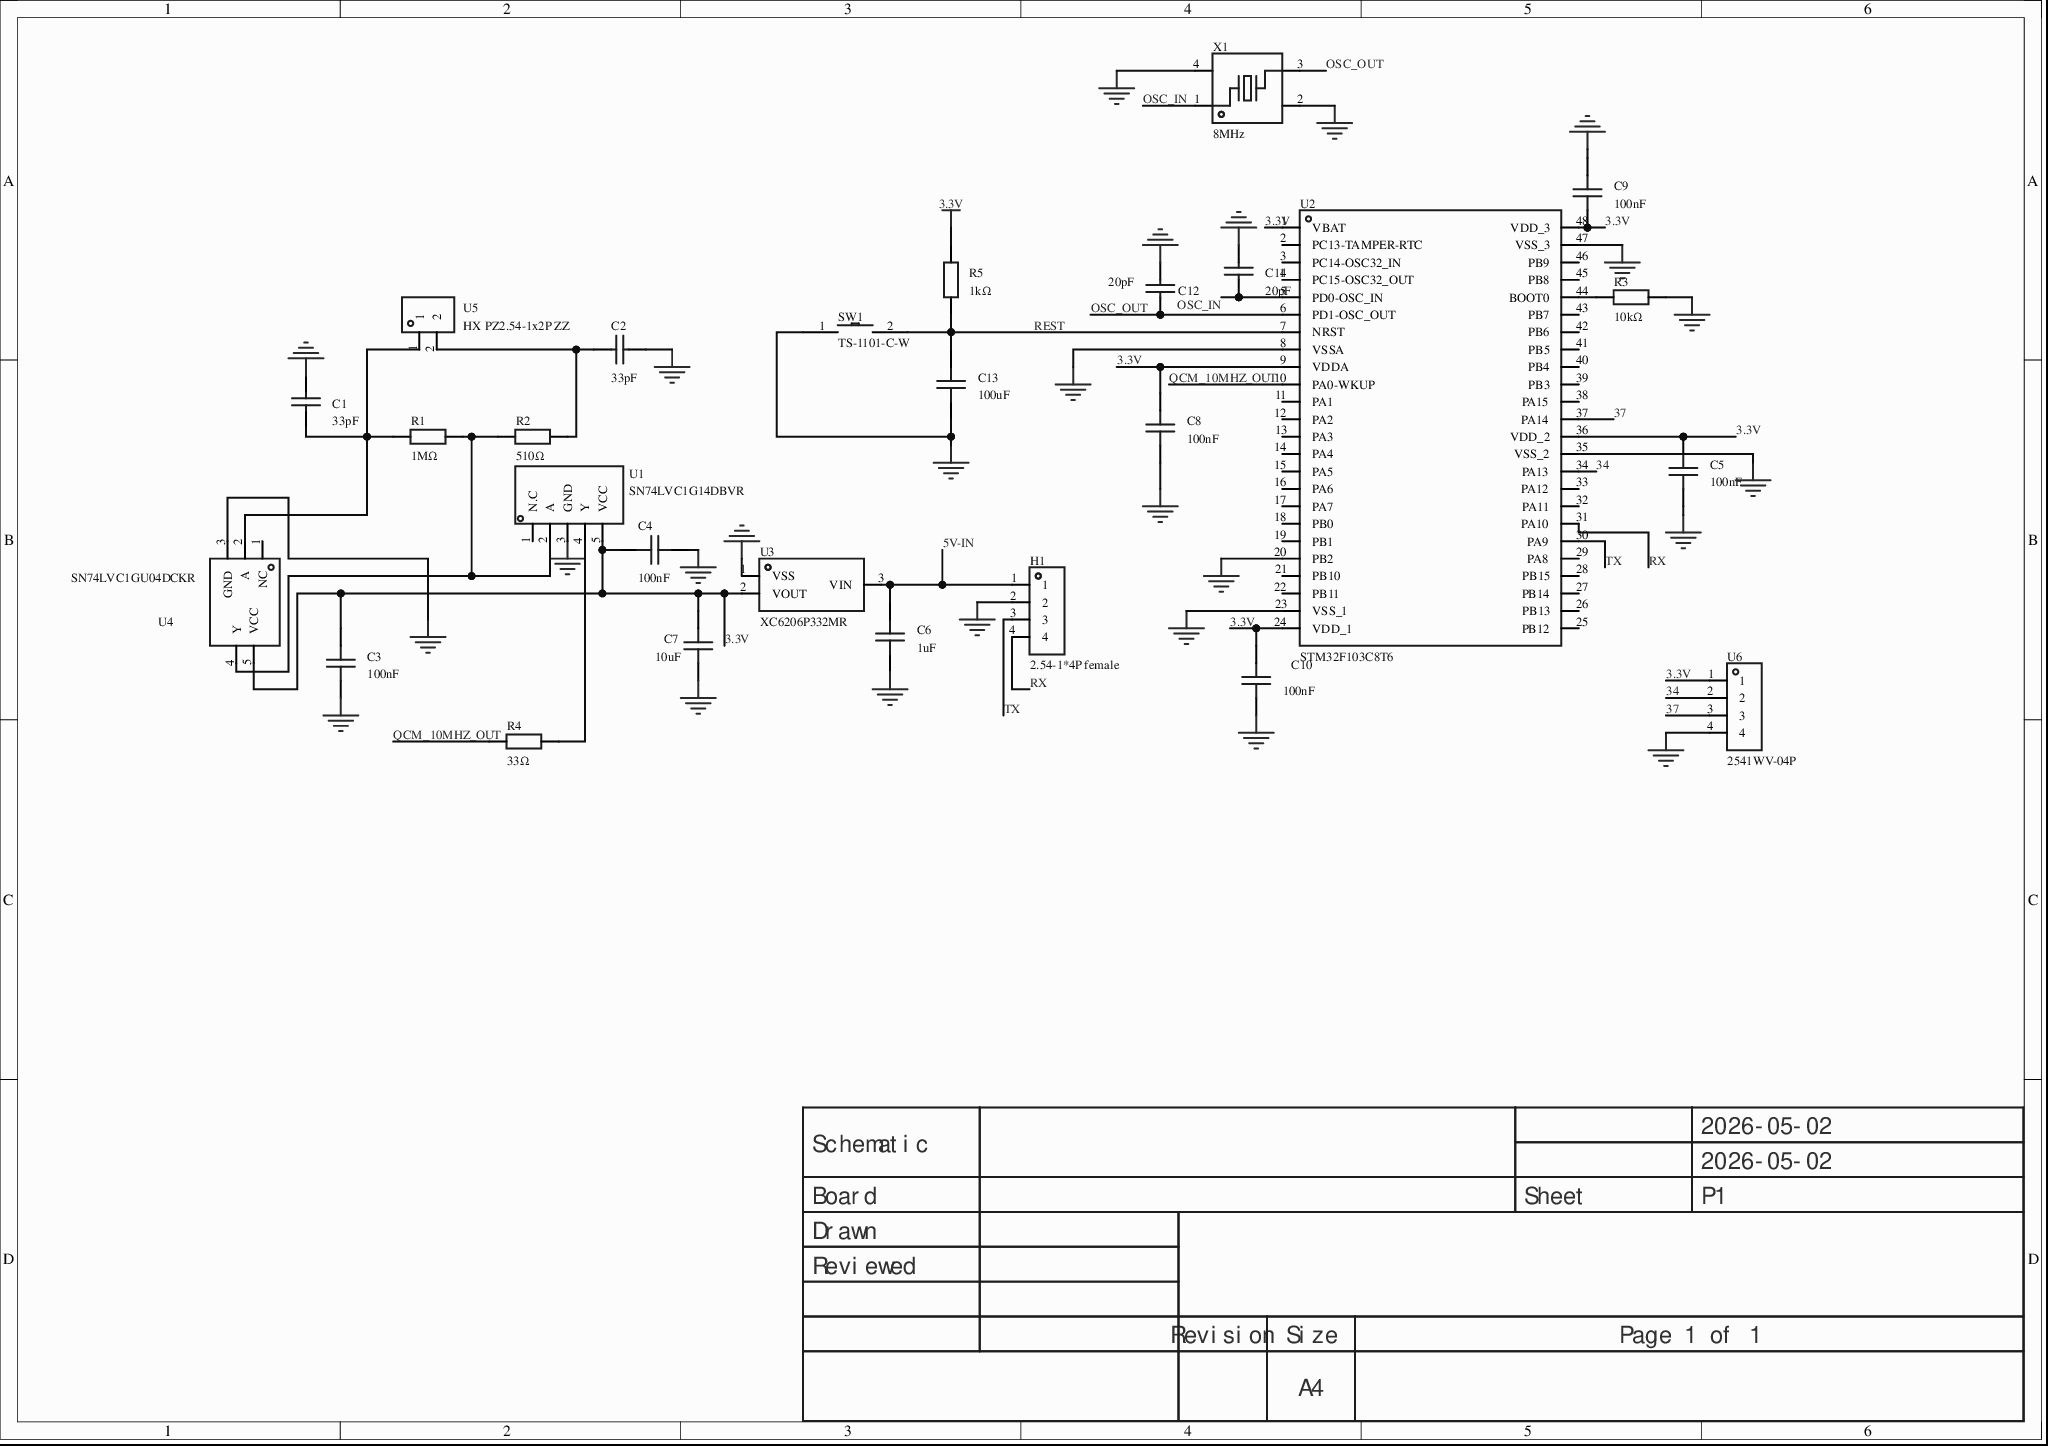
[diagram p0: MISC51896-3.schdoc]
# Altium project MISC51896-2.PrjPcb
1 sheet, 27 parts. Net scope: global (net labels, ports and power ports of the same name join across sheets).
Board file: MISC51896.pcbdoc

## Sheet MISC51896-3.schdoc
size 297 x 209 mm; Version: V1.0; @Project Name: MISC51896; @Update Date: 2026-05-02; @Create Date: 2026-05-02; @Board Name: MISC51896; @Create Time: 19:24:28; @Page Count: 1; @Page No: 1; @Schematic Name: MISC51896; @Update Time: 19:24:28; Size: A4

### Parts
C1  33pF  [C0603]
C2  33pF  [C0603]
C3  100nF  [C0603]
C4  100nF  [C0603]
C5  100nF  [C0603]
C6  1uF  [C0603]
C7  10uF  [C0603]
C8  100nF  [C0603]
C9  100nF  [C0603]
C10  100nF  [C0603]
C11  20pF  [C0603]
C12  20pF  [C0603]
C13  100uF  [C1206]
H1  2.54-1*4P female  [HDR-TH_4P-P2.54-V-F]
R1  1MΩ  [R0603]
R2  510Ω  [R0603]
R3  10kΩ  [R0603]
R4  33Ω  [R0603]
R5  1kΩ  [R0603]
SW1  TS-1101-C-W  [SW-SMD_L6.0-W3.3-LS8.0]
U1  SN74LVC1G14DBVR  [SOT-23-5_L3.0-W1.7-P0.95-LS2.8-BR]
U2  STM32F103C8T6  [LQFP-48_L7.0-W7.0-P0.50-LS9.0-BL]
U3  XC6206P332MR  [SOT-23-3_L3.0-W1.7-P0.95-LS2.9-BR]
U4  SN74LVC1GU04DCKR  [SC-70-5_L2.1-W1.3-P0.65-LS2.1-BL]
U5  HX PZ2.54-1x2P ZZ  [HDR-TH_2P-P2.54-V-M-3]
U6  2541WV-04P  [HDR-TH_4P-P2.54-V-M-1]
X1  8MHz  [CRYSTAL-SMD_4P-L3.2-W2.5-BL]

### Nets
3.3V: C3.2 C4.1 C5.2 C7.2 C8.2 C9.1 C10.2 R5.2 U1.5(VCC) U2.1(VBAT) U2.9(VDDA) U2.24(VDD_1) U2.36(VDD_2) U2.48(VDD_3) U3.2(VOUT) U4.5(VCC) U6.1
GND: C1.2 C2.2 C3.1 C4.2 C5.1 C6.1 C7.1 C8.1 C9.2 C10.1 C11.2 C12.2 C13.1 H1.2 R3.2 SW1.1 U1.3(GND) U2.8(VSSA) U2.20(PB2) U2.23(VSS_1) U2.35(VSS_2) U2.47(VSS_3) U3.1(VSS) U4.3(GND) U6.4 X1.2(GND) X1.4(GND)
5V-IN: C6.2 H1.1 U3.3(VIN)
34: U2.34(PA13) U6.2
37: U2.37(PA14) U6.3
OSC_IN: C11.1 U2.5(PD0-OSC_IN) X1.1
OSC_OUT: C12.1 U2.6(PD1-OSC_OUT) X1.3
QCM_10MHZ_OUT: R4.1 U2.10(PA0-WKUP)
REST: C13.2 R5.1 SW1.2 U2.7(NRST)
RX: H1.4 U2.31(PA10)
TX: H1.3 U2.30(PA9)
NetC1_1: C1.1 R1.1 U4.2(A) U5.1
NetC2_1: C2.1 R2.2 U5.2
NetR1_2: R1.2 R2.1 U1.2(A) U4.4(Y)
NetR3_1: R3.1 U2.44(BOOT0)
NetR4_2: R4.2 U1.4(Y)

Not connected (* = marked no-connect by the designer): U1 1(N.C); U2 2(PC13-TAMPER-RTC) 3(PC14-OSC32_IN) 4(PC15-OSC32_OUT) 11(PA1) 12(PA2) 13(PA3) 14(PA4) 15(PA5) 16(PA6) 17(PA7) 18(PB0) 19(PB1) 21(PB10) 22(PB11) 25(PB12) 26(PB13) 27(PB14) 28(PB15) 29(PA8) 32(PA11) 33(PA12) 38(PA15) 39(PB3) 40(PB4) 41(PB5) 42(PB6) 43(PB7) 45(PB8) 46(PB9); U4 1(NC)

### Notes on the sheet
- 2026-05-02
- Schematic
- Board
- Sheet
- P1
- Drawn
- Reviewed
- Revision
- Size
- A4
- Page 1 of 1

### Library data of the parts
C1 C2 = CL10C330JB8NNNC: Capacitance:33pF;Tolerance:±5%;Rated voltage:50V;Temperature coefficient:C0G;; Manufacturer: SAMSUNG(三星); AddInBom: yes; ModelId: ac125912035d415993ca9572d50418b10819f05c4eef4c71ace90d822a990e87; ModelName: C0603_L1.6-W0.8-H0.8; ModelTransform: 62.992,31.496,0,0,0,0,0,0,0; Tolerance: ±5%; Voltage Rating: 50V; Temperature Coefficient: C0G; Symbol: CL10C330JB8NNNC; Device: CL10C330JB8NNNC; LCSC Part Name: 33pF ±5% 50V; SupplierPart: C1663; ManufacturerPart: CL10C330JB8NNNC; Supplier Footprint: 0603; JLCPCB Part Class: Basic Part; Datasheet: https://item.szlcsc.com/datasheet/CL10C330JB8NNNC/2015.html; Supplier: LCSC; ConvertToPcb: yes; FootprintName: C0603; Value: 33pF
C3 C4 = CGA0603X7R104K500JT: Capacitance:100nF;Tolerance:±10%;Rated voltage:50V;Temperature coefficient:X7R;; Manufacturer: HRE(芯声); AddInBom: yes; ModelId: ac125912035d415993ca9572d50418b10819f05c4eef4c71ace90d822a990e87; ModelName: C0603_L1.6-W0.8-H0.8; ModelTransform: 62.992,31.496,0,0,0,0,0,0,0; Tolerance: ±10%; Voltage Rating: 50V; Temperature Coefficient: X7R; Symbol: CGA0603X7R104K500JT; Device: CGA0603X7R104K500JT; LCSC Part Name: 100nF ±10% 50V; SupplierPart: C6119867; ManufacturerPart: CGA0603X7R104K500JT; Supplier Footprint: 0603; JLCPCB Part Class: Extended Part; Datasheet: https://item.szlcsc.com/datasheet/CGA0603X7R104K500JT/7062573.html; Supplier: LCSC; ConvertToPcb: yes; FootprintName: C0603; Value: 100nF
C5 C8-C10 = CGA0603X7R104K500JT: Capacitance:100nF;Tolerance:±10%;Rated voltage:50V;Temperature coefficient:X7R;; Manufacturer: HRE(芯声); Add into BOM: yes; 3D Model: ac125912035d415993ca9572d50418b1; 3D Model Transform: 62.992,31.496,0,0,0,0,0,0,0; Tolerance: ±10%; Voltage Rating: 50V; Temperature Coefficient: X7R; ModelName: C0603_L1.6-W0.8-H0.8; Symbol: CGA0603X7R104K500JT; Device: CGA0603X7R104K500JT; Convert to PCB: yes; LCSC Part Name: 100nF ±10% 50V; Supplier Part: C6119867; Manufacturer Part: CGA0603X7R104K500JT; Supplier Footprint: 0603; JLCPCB Part Class: Extended Part; Datasheet: https://item.szlcsc.com/datasheet/CGA0603X7R104K500JT/7062573.html; Supplier: LCSC; Value: 100nF; FootprintName: C0603
C6 C7 = CGA0603X5R105K500JT: Capacitance:1uF;Tolerance:±10%;Rated voltage:50V;Temperature coefficient:X5R;; Manufacturer: HRE(芯声); AddInBom: yes; ModelId: ac125912035d415993ca9572d50418b10819f05c4eef4c71ace90d822a990e87; ModelName: C0603_L1.6-W0.8-H0.8; ModelTransform: 62.992,31.496,0,0,0,0,0,0,0; Tolerance: ±10%; Voltage Rating: 50V; Temperature Coefficient: X5R; Symbol: CGA0603X5R105K500JT; Device: CGA0603X5R105K500JT; LCSC Part Name: 1uF ±10% 50V; ManufacturerPart: CGA0603X5R105K500JT; Supplier Footprint: 0603; JLCPCB Part Class: Extended Part; Datasheet: https://item.szlcsc.com/datasheet/CGA0603X5R105K500JT/7062558.html; Supplier: LCSC; ConvertToPcb: yes; FootprintName: C0603
  C6: SupplierPart: C6119852; Value: 1uF
  C7: Value: 10uF
C11 C12 = CL10C200JB8NNNC: Capacitance:20pF;Tolerance:±5%;Rated voltage:50V;Temperature coefficient:C0G;; Manufacturer: SAMSUNG(三星); Add into BOM: yes; 3D Model: ac125912035d415993ca9572d50418b1; 3D Model Transform: 62.992,31.496,0,0,0,0,0,0,0; Tolerance: ±5%; Voltage Rating: 50V; Temperature Coefficient: C0G; ModelName: C0603_L1.6-W0.8-H0.8; Symbol: CL10C200JB8NNNC; Device: CL10C200JB8NNNC; Convert to PCB: yes; Supplier Footprint: 0603; Value: 20pF; LCSC Part Name: 20pF ±5% 50V; Supplier Part: C1648; Manufacturer Part: CL10C200JB8NNNC; JLCPCB Part Class: Basic Part; Datasheet: https://item.szlcsc.com/datasheet/CL10C200JB8NNNC/2000.html; Supplier: LCSC; FootprintName: C0603
C13 = HGC1206R5107M100NSPJ: Capacitance:100uF;Tolerance:±20%;Rated voltage:10V;Dielectric (temperature coefficient):X5R;; Manufacturer: Chinocera(华瓷); 3D Model: e4be705b945545a48e666415e3682bd8; 3D Model Transform: 125.984,62.992,0,0,0,0,0,0,0; Tolerance: ±20%; Voltage Rated: 10V; Temperature Coefficient: X5R; AddInBom: yes; ModelName: C1206_L3.2-W1.6-H1.3; Symbol: HGC1206R5107M100NSPJ; Device: HGC1206R5107M100NSPJ; LCSC Part Name: 100uF ±20% 10V; Supplier Part: C7432784; Manufacturer Part: HGC1206R5107M100NSPJ; Supplier Footprint: 1206; JLCPCB Part Class: Extended library; Datasheet: https://atta.szlcsc.com/upload/public/pdf/source/20240320/FAC3FEC40A78BC5CCCE96C232A94D860.pdf; Supplier: LCSC; Value: 100uF; ConvertToPcb: yes; FootprintName: C1206
H1 = 2.54-1*4P母: Socket structure:1x4P;Pitch:2.54mm;Row spacing:-;Round/square hole:square hole;Mounting:through-hole;Rows:single row;Total holes:4P;Rated current:3A;Rated voltage:-;Socket direction:top;Plastic height:-;Contact material:Bronze;Contact plating:-;Operating temperature:-40℃~+105℃;; Manufacturer: BOOMELE(博穆精密); AddInBom: yes; ModelId: d187812051054f85879fcaa51a310d8e0819f05c4eef4c71ace90d822a990e87; ModelTransform: 419.6842,98.464,0,0,0,0,0,0,-118.11; Holes Structure: 1x4P; Pitch: 2.54mm; Number of Positions: 4P; Current Rating: 3A; Holes Direction: Top; Symbol: 2.54-1*4P female; Device: 2.54-1*4P female; LCSC Part Name: 间距:2.54mm 1x4P 直插; SupplierPart: C2718488; ManufacturerPart: 2.54-1*4P母; Supplier Footprint: 插件,P=2.54mm; JLCPCB Part Class: Extended Part; Datasheet: https://item.szlcsc.com/datasheet/2.54-1*4P%25E6%25AF%258D/2834502.html; Supplier: LCSC; ConvertToPcb: yes; FootprintName: HDR-TH_4P-P2.54-V-F; ModelName: HDR-TH_4P-P2.54-V-F; Row Spacing: -; Circular Hole / Square Hole: Square hole; Mounting Type: Through-hole; Number of Rows: Single row; Voltage Rating (Max): -; Insulation Height: -; Contact Material: Bronze; Contact Plating: -; Operating Temperature: -40℃~+105℃
R1 = 0603WAF1004T5E: Resistor type:thick film;Resistance:1MΩ;Tolerance:±1%;Power:100mW;Max working voltage:75V;Temperature coefficient:±100ppm/℃;; Manufacturer: UNI-ROYAL(厚声); AddInBom: yes; ModelId: fc143cca1e79419f9cd78b61e9279f080819f05c4eef4c71ace90d822a990e87; ModelTransform: 31.8897,63.7794,0,90,0,0,0,0,0; Tolerance: ±1%; Power(Watts): 100mW; Overload Voltage (Max): 75V; Symbol: 0603WAF1004T5E; Device: 0603WAF1004T5E; LCSC Part Name: 1MΩ ±1% 100mW 厚膜电阻; SupplierPart: C22935; ManufacturerPart: 0603WAF1004T5E; Supplier Footprint: 0603; JLCPCB Part Class: Basic Part; Datasheet: https://atta.szlcsc.com/upload/public/pdf/source/20200306/C422600_1E6D84923E4A46A82E41ADD87F860B5C.pdf; Supplier: LCSC; ConvertToPcb: yes; FootprintName: R0603; ModelName: R0603; Type: Thick film resistor; Value: 1MΩ; Temperature Coefficient: ±100ppm/℃; Operating Temperature Range: -55℃~+155℃
R2 = 0603WAF5100T5E: Resistor type:thick film;Resistance:510Ω;Tolerance:±1%;Power:100mW;Working voltage:75V;Temperature coefficient:±100ppm/℃;; Manufacturer: UNI-ROYAL(厚声); Add into BOM: yes; 3D Model: fc143cca1e79419f9cd78b61e9279f08; 3D Model Transform: 31.8897,63.7794,0,90,0,0,0,0,0; Tolerance: ±1%; Power(Watts): 100mW; Voltage-Supply(Max): 75V; Symbol: 0603WAF5100T5E; Device: 0603WAF5100T5E; Convert to PCB: yes; LCSC Part Name: 510Ω ±1% 100mW 厚膜电阻; Supplier Part: C23193; Manufacturer Part: 0603WAF5100T5E; Supplier Footprint: 0603; JLCPCB Part Class: Basic Part; Datasheet: https://item.szlcsc.com/datasheet/0603WAF5100T5E/23920.html; Supplier: LCSC; Type: Thick film resistor; Value: 510Ω; Temperature Coefficient: ±100ppm/℃; Operating Temperature: -55℃~+155℃; FootprintName: R0603; ModelName: R0603
R3 R4 = Res_0603: Symbol: Resistor; ConvertToPcb: yes; ModelId: fc143cca1e79419f9cd78b61e9279f080819f05c4eef4c71ace90d822a990e87; ModelTransform: 31.8897,63.7794,0,90,0,0,0,0,0; Device: Res_0603; AddInBom: yes; Supplier Footprint: 0603; FootprintName: R0603; ModelName: R0603
  R3: Value: 10kΩ
  R4: Value: 33Ω
R5 = RC0603FR-071KL: Resistor type:thick film;Resistance:1kΩ;Tolerance:±1%;Power:100mW;Max working voltage:75V;Temperature coefficient:±100ppm/℃;; Manufacturer: YAGEO(国巨); 3D Model: fc143cca1e79419f9cd78b61e9279f08; 3D Model Transform: 31.8897,63.7794,0,90,0,0,0,0,0; Tolerance: ±1%; Power(Watts): 100mW; Overload Voltage (Max): 75V; AddInBom: yes; Symbol: RC0603FR-071KL; Device: RC0603FR-071KL; LCSC Part Name: 厚膜电阻 1kΩ ±1% 100mW; Supplier Part: C22548; Manufacturer Part: RC0603FR-071KL; Supplier Footprint: 0603; JLCPCB Part Class: Extended library; Datasheet: https://atta.szlcsc.com/upload/public/pdf/source/20180316/70C0E2BDAE7FCC62C531A5A58D202EE1.pdf; Supplier: LCSC; Type: Thick film resistor; Value: 1kΩ; Temperature Coefficient: ±100ppm/℃; Operating Temperature Range: -55℃~+155℃; ConvertToPcb: yes; FootprintName: R0603; ModelName: R0603
SW1 = TS-1101-C-W: Circuit:SPST;Button shape:rectangular button;Actuating force:260gf;Mounting:surface mount;Switch length:6mm;Switch width:3.6mm;Switch height:2.5mm;Bracket:none;Contact current:50mA;Rated voltage (AC):-;Rated voltage (DC):12V;Rated power:-;Insulation resistance:-;Lamp:none;Mechanical life:5万 cycles;; Manufacturer: XKB Connectivity(中国星坤); 3D Model: b2f4ea9f0afc4b0786d53dba66ceb9e4; 3D Model Transform: 314.96,129.921,0,0,0,0,0,0,0; Circuit: SPST; Operating Force: 260gf; Switch Length: 6mm; Switch Width: 3.6mm; Switch Height: 2.5mm; Strike Gundam: Without bracket; Contact Current: 50mA; Voltage Rating (DC): 12V; Actuator/Cap Color: White with light green tint; With Lamp: None; AddInBom: yes; ModelName: SW-SMD_L6.0-W3.3-H5-LS8.0; Symbol: TS-1101-C-W; Device: TS-1101-C-W; LCSC Part Name: 6*3.6*2.5mm 立贴 轻触开关; Supplier Part: C318938; Manufacturer Part: TS-1101-C-W; Supplier Footprint: SMD; JLCPCB Part Class: Extended library; Datasheet: https://atta.szlcsc.com/upload/public/pdf/source/20200227/C318938_C2E53B1EEDE37D980A33616AC086DE53.pdf; Supplier: LCSC; Actuator Style: Rectangular button; Mounting Style: Surface mount; Voltage Rating (AC): -; Power Rating: -; Insulation Resistance: -; IP Rating: -; Pin Style: -; Mechanical Life: 5万 cycles; Operating Temperature: -30℃~+85℃; ConvertToPcb: yes; FootprintName: SW-SMD_L6.0-W3.3-LS8.0
U1 = SN74LVC1G14DBVR: Input type:Schmitt trigger;Operating voltage:1.65V~5.5V;Quiescent current (Iq):10uA;Channels:1;Propagation delay (tpd):6.5ns@2.5V,50pF;; Manufacturer: TI(德州仪器); AddInBom: yes; ModelId: 0a2a1b8f50944f73965918ad6e5fe1670819f05c4eef4c71ace90d822a990e87; ModelName: SOT-23-5_L2.9-W1.6-H1.1-LS2.8-P0.95; ModelTransform: 114.173,109.636,0,180,0,0,0,0,0; Quiescent Current(Iq): 10uA; Number of Circuits: 1; Current - Output Low(IOL): 32mA; Input Logic Level - High: 1.16V~3.33V; Input Logic Level -Low: 390mV~1.87V; Output Logic Level - High: 2.3V; Output Logic Level - Low: 550mV; Symbol: SN74LVC1G14DBVR; Device: SN74LVC1G14DBVR; LCSC Part Name: 单路施密特触发反相器; SupplierPart: C7835; ManufacturerPart: SN74LVC1G14DBVR; Supplier Footprint: SOT-23-5; JLCPCB Part Class: Extended Part; Supplier: LCSC; ConvertToPcb: yes; FootprintName: SOT-23-5_L3.0-W1.7-P0.95-LS2.8-BR; Input Type: Schmitt trigger; Voltage - Supply: 1.65V~5.5V; Number of Inputs: 1; Current - Output High(IOH): 32mA; Propagation Delay: 6.5ns@2.5V,50pF; Series: 74LVC series; Operating Temperature: -40℃~+85℃
U2 = STM32F103C8T6: CPU core:ARM-M3;Max CPU frequency:72MHz;Application field:-;; Manufacturer: ST(意法半导体); AddInBom: yes; ModelId: 093be70396ff421eb2cdb946d5311efc0819f05c4eef4c71ace90d822a990e87; ModelName: LQFP-48_L7.0-W7.0-H1.4-LS9.0-P0.50; ModelTransform: 354.331,354.331,0,0,0,0,0,0,0; CPU Core: ARM-M3; CPU Maximum Speed: 72MHz; Program Storage Size: 64KB; Program Memory Type: FLASH; Number of I/O: 37; ADC (Bit): 12bit; Voltage - Supply: 2V~3.6V; Symbol: STM32F103C8T6; Device: STM32F103C8T6; LCSC Part Name: 主流增强型ARM Cortex-M3 MCU，具有64 KB Flash、72 MHz CPU、电机控制、USB和CAN; SupplierPart: C8734; ManufacturerPart: STM32F103C8T6; Supplier Footprint: LQFP-48(7x7); JLCPCB Part Class: Extended Part; Datasheet: https://item.szlcsc.com/datasheet/STM32F103C8T6/9243.html; Supplier: LCSC; ConvertToPcb: yes; FootprintName: LQFP-48_L7.0-W7.0-P0.50-LS9.0-BL; Applications: -
U3 = XC6206P332MR_C347376: Output type:fixed;Operating voltage:8V;Output voltage:3.3V;Output current:250mA;Ripple rejection (PSRR):40dB@(1kHz);Output polarity:positive;; Manufacturer: UMW(友台半导体); AddInBom: yes; ModelId: 89cb27a44ab2466697082bb9fd73a7d00819f05c4eef4c71ace90d822a990e87; ModelName: SOT-23-3L_L2.9-W1.6-H1.1-LS2.8-P0.95; ModelTransform: 114.173,110.236,0,90,0,0,0,0,0; Output Type: Fixed; Voltage - Supply: 8V; Output Voltage: 3.3V; Output Current: 250mA; Voltage Dropout: 240mV@(50mA); standby current: 7uA; Number of Outputs: 1; Symbol: XC6206P332MR_C347376; Device: XC6206P332MR_C347376; LCSC Part Name: 高纹波抑制率、低功耗、低压差 CMOS 降压型电压稳压器; SupplierPart: C347376; ManufacturerPart: XC6206P332MR; Supplier Footprint: SOT-23; JLCPCB Part Class: Extended Part; Datasheet: https://item.szlcsc.com/datasheet/XC6206P332MR/324036.html; Supplier: LCSC; ConvertToPcb: yes; FootprintName: SOT-23-3_L3.0-W1.7-P0.95-LS2.9-BR; Power Supply Rejection Ratio (PSRR): 40dB@(1kHz); Noise: -; Features: Overcurrent protection; short-circuit protection; Operating Temperature: -25℃~+80℃@(Ta); Output Configuration: Positive
U4 = SN74LVC1GU04DCKR: Input type:-;Operating voltage:1.65V~5.5V;Quiescent current (Iq):10uA;Channels:1;Propagation delay (tpd):3.5ns@5V,50pF;; Manufacturer: TI(德州仪器); AddInBom: yes; ModelId: c1de3ed719554bdea19f5a56956153530819f05c4eef4c71ace90d822a990e87; ModelName: SC-70-5_L2.0-W1.3-H1.0-P0.65; ModelTransform: 82.677,78.74,0,90,0,0,0,0,0; Quiescent Current(Iq): 10uA; Number of Circuits: 1; Current - Output Low(IOL): 32mA; Input Logic Level - High: 1.24V~4.13V; Input Logic Level -Low: 410mV~1.38V; Symbol: SN74LVC1GU04DCKR; Device: SN74LVC1GU04DCKR; LCSC Part Name: 单路反相器; SupplierPart: C485082; ManufacturerPart: SN74LVC1GU04DCKR; Supplier Footprint: SC-70-5; JLCPCB Part Class: Extended Part; Supplier: LCSC; ConvertToPcb: yes; FootprintName: SC-70-5_L2.1-W1.3-P0.65-LS2.1-BL; Input Type: -; Voltage - Supply: 1.65V~5.5V; Number of Inputs: 1; Current - Output High(IOH): 32mA; Output Logic Level - High: -; Output Logic Level - Low: -; Propagation Delay: 3.5ns@5V,50pF; Series: 74LVC series; Operating Temperature: -40℃~+125℃
U5 = HX PZ2.54-1x2P ZZ: Pin structure:1x2P;Pitch:2.54mm;Row spacing:-;Round/square pin:square pin;Mounting:through-hole;Rows:single row;Total pins:2P;Rated current:3A;Rated voltage:1kV;Mating pin length:6mm;Plastic height:2.5mm;Termination pin length:3mm;Contact material:Brass;Contact plating:Gold;Operating temperature:-40℃~+105℃;Color:black;; Manufacturer: hanxia(韩下); AddInBom: yes; ModelId: c7a9f3c3e6e34627af2bf939e464cb350819f05c4eef4c71ace90d822a990e87; ModelName: HDR-TH_2P-P2.54-M-LI-1X2P; ModelTransform: 200,100,0,0,0,0,0,0,-118.11; Pin Structure: 1x2P; Pitch: 2.54mm; Current Rating: 3A; Voltage Rating (Max): 1kV; Symbol: HX PZ2.54-1X2P ZZ; Device: HX PZ2.54-1x2P ZZ; LCSC Part Name: 1x2P 间距:2.54mm 方针 直插; SupplierPart: C32713268; ManufacturerPart: HX PZ2.54-1x2P ZZ; Supplier Footprint: 插件,P=2.54mm; JLCPCB Part Class: Extended Part; Datasheet: https://item.szlcsc.com/datasheet/HX%2520PZ2.54-1x2P%2520ZZ/34444548.html; Supplier: LCSC; ConvertToPcb: yes; FootprintName: HDR-TH_2P-P2.54-V-M-3; Row Spacing: -; Circluar Pins/Square Pins: Square pin; Mounting Type: Through-hole; Number of Rows: Single row; Number of Pins: 2P; Length of Mating Pin: 6mm; Insulation Height: 2.5mm; Length of End Connection Pin: 3mm; Contact Material: Brass; Contact Plating: Gold; Operating Temperature: -40℃~+105℃; Color: Black; Supplementary Features: -
U6 = 2541WV-04P: Pin structure:1x4P;Pitch:2.54mm;Row spacing:-;Round/square pin:square pin;Mounting:through-hole;Rows:single row;Total pins:4P;Rated current:3A;Mating pin length:6mm;Plastic height:2.54mm;Termination pin length:3mm;Contact material:Brass;Contact plating:Gold;Operating temperature:-55℃~+105℃;; Manufacturer: HanElectricity(瀚源); AddInBom: yes; ModelId: e2e03939c192453cba872779c0cb63900819f05c4eef4c71ace90d822a990e87; ModelTransform: 400.039,100,0,0,0,0,0,0,-118.11; Pin Structure: 1x4P; Pitch: 2.54mm; Current Rating: 3A; Symbol: 2541WV-04P; Device: 2541WV-04P; LCSC Part Name: 1x4P 间距:2.54mm 方针 直插; SupplierPart: C5383113; ManufacturerPart: 2541WV-04P; Supplier Footprint: 插件,P=2.54mm; JLCPCB Part Class: Extended Part; Datasheet: https://item.szlcsc.com/datasheet/2541WV-04P/6258473.html; Supplier: LCSC; ConvertToPcb: yes; FootprintName: HDR-TH_4P-P2.54-V-M-1; ModelName: HDR-TH_4P-P2.54-V-M-1; Row Spacing: -; Circluar Pins/Square Pins: Square pin; Mounting Type: Through-hole; Number of Rows: Single row; Number of Pins: 4P; Length of Mating Pin: 6mm; Insulation Height: 2.54mm; Length of End Connection Pin: 3mm; Contact Material: Brass; Contact Plating: Gold; Operating Temperature: -55℃~+105℃
X1 = X32258MSB4SI: Crystal type:SMD crystal;Frequency:8MHz;Tolerance at room temperature:±10ppm;Load capacitance:20pF;Frequency stability:±20ppm;; Manufacturer: YXC(扬兴晶振); AddInBom: yes; ModelId: ff2dfd5650294453a14147960efe18380819f05c4eef4c71ace90d822a990e87; ModelTransform: 125.984,98.425,0,0,0,0,0,0,0; Normal temperature Frequency Tolerance: ±10ppm; Load Capacitance: 20pF; Frequency Stability: ±20ppm; Equivalent Series Resistance(ESR): 120Ω; Symbol: X32258MSB4SI; Device: X32258MSB4SI; LCSC Part Name: YSX321SL 8MHZ 4P 3225 20PF ±10PPM -40~85℃ (±20PPM); SupplierPart: C2682774; ManufacturerPart: X32258MSB4SI; Supplier Footprint: SMD3225-4P; JLCPCB Part Class: Extended Part; Datasheet: https://item.szlcsc.com/datasheet/X32258MSB4SI/2777871.html; Supplier: LCSC; ConvertToPcb: yes; FootprintName: CRYSTAL-SMD_4P-L3.2-W2.5-BL; ModelName: CRYSTAL-SMD_4P-L3.2-W2.5-BL; Type: SMD crystal; Value: 8MHz; Operating Temperature: -40℃~+85℃